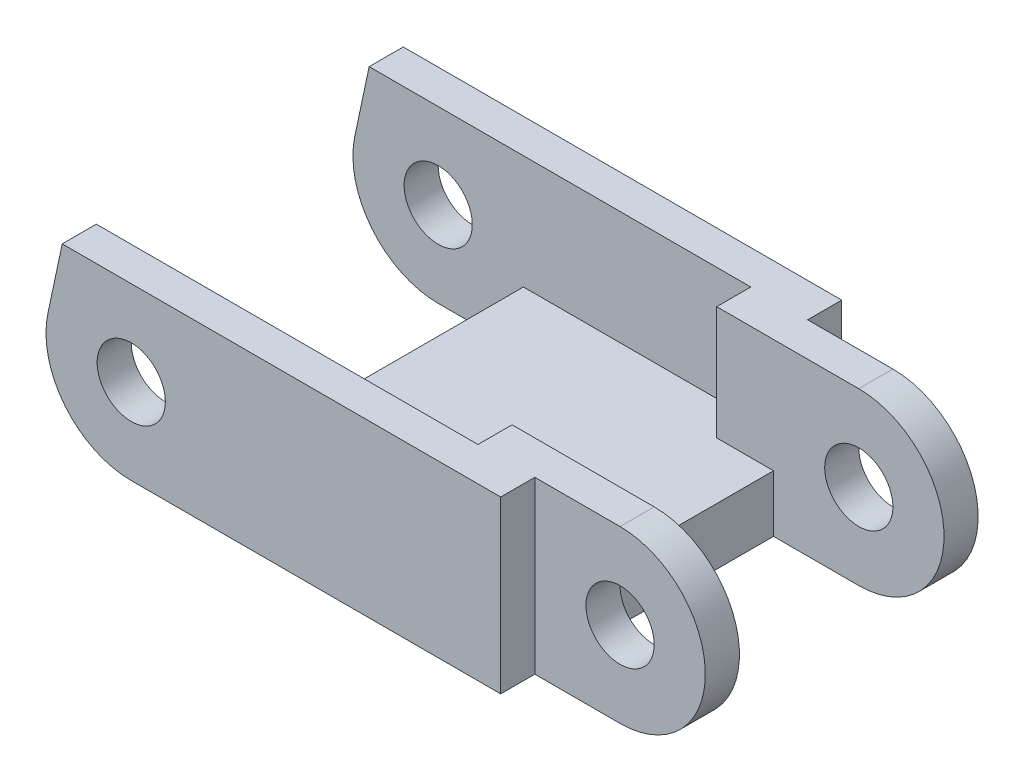
from build123d import *

# Parameters (mm, degrees)
SKETCH1_R           = 3
BOSS_EXTRUDE1_DEPTH = 30
SKETCH2_W           = 30
SKETCH2_H           = 24
SKETCH2_H_2         = 6
CUT_EXTRUDE1_DEPTH  = 30
CUT_EXTRUDE2_DEPTH  = 10
SKETCH4_W           = 29.142135624
SKETCH4_H           = 18
CUT_EXTRUDE3_DEPTH  = 12


with BuildPart() as part:
    # Sketch1 → Boss-Extrude1 (new body)
    with BuildSketch(Plane.XY):
        with BuildLine():
            Line((1.925621669, 9.059337681), (3.188348425, 15))
            Line((3.188348425, 15), (49.261728674, 15))
            ThreePointArc((49.261728674, 15), (56.761728674, 7.5), (49.261728674, 0))
            Line((49.261728674, 0), (9.261728674, 0))
            ThreePointArc((9.261728674, 0), (3.433133963, 2.780097067), (1.925621669, 9.059337681))
        make_face()
        with Locations((9.261728674, 7.5)):
            Circle(SKETCH1_R, mode=Mode.SUBTRACT)
        with Locations((49.261728674, 7.5)):
            Circle(SKETCH1_R, mode=Mode.SUBTRACT)
    extrude(amount=BOSS_EXTRUDE1_DEPTH)

    # Sketch2 → Cut-Extrude1 (cut)
    with BuildSketch(Plane(origin=(0, 15, 0), x_dir=(1, 0, 0), z_dir=(0, 1, 0))):
        with Locations((1.761728674, -15)):
            Rectangle(SKETCH2_W, SKETCH2_H)
        with Locations((56.761728674, 0)):
            Rectangle(SKETCH2_W, SKETCH2_H_2)
        with Locations((56.761728674, -30)):
            Rectangle(SKETCH2_W, SKETCH2_H_2)
    extrude(amount=-CUT_EXTRUDE1_DEPTH, mode=Mode.SUBTRACT)

    # Sketch3 → Cut-Extrude2 (cut)
    with BuildSketch(Plane(origin=(0, 15, 0), x_dir=(1, 0, 0), z_dir=(0, 1, 0))):
        Polygon((-3.238271326, -3), (36.761728674, -3), (36.761728674, -6), (65.37522755, -6), (65.37522755, -24), (36.761728674, -24), (36.761728674, -27), (-3.238271326, -27), align=None)
    extrude(amount=-CUT_EXTRUDE2_DEPTH, mode=Mode.SUBTRACT)

    # Sketch4 → Cut-Extrude3 (cut)
    with BuildSketch(Plane(origin=(0, 5, 0), x_dir=(1, 0, 0), z_dir=(0, 1, 0))):
        with Locations((56.332796486, -15)):
            Rectangle(SKETCH4_W, SKETCH4_H)
    extrude(amount=-CUT_EXTRUDE3_DEPTH, mode=Mode.SUBTRACT)


solid = part.part
